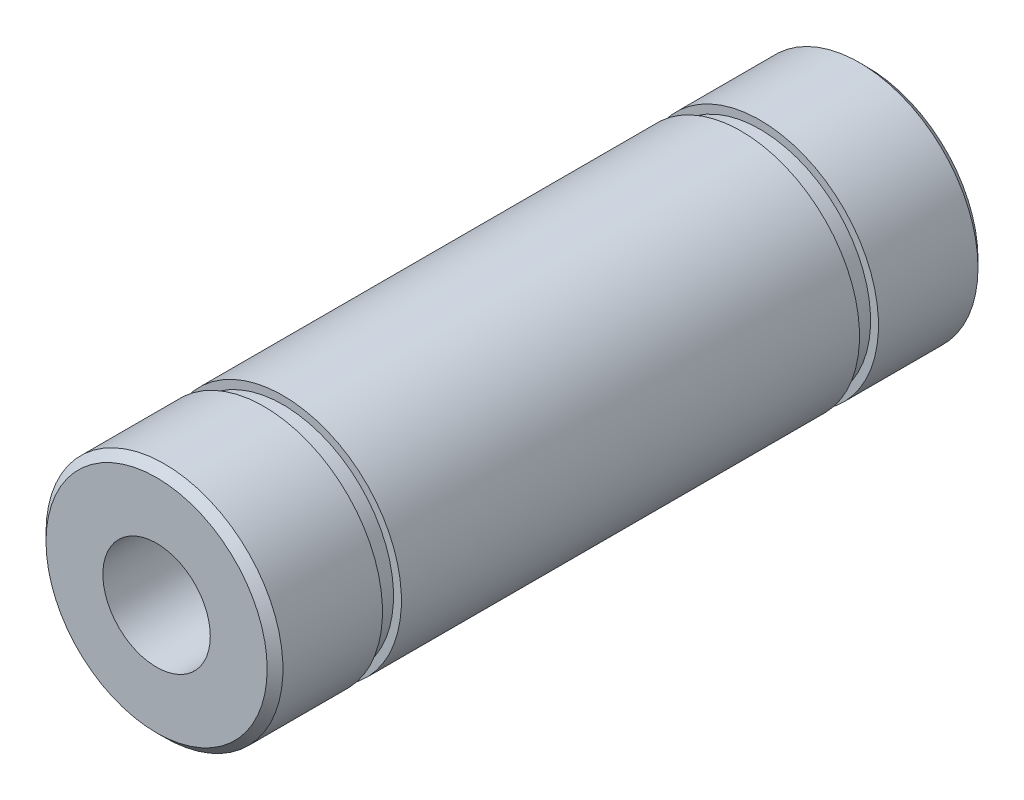
SolidWorks part; units mm, degrees
ref_plane "前视" through (0, 0, 0) normal (0, 0, 1) x (1, 0, 0)
ref_plane "上视" through (0, 0, 0) normal (0, 1, 0) x (1, 0, 0)
ref_plane "右视" through (0, 0, 0) normal (1, 0, 0) x (0, 0, -1)
sketch "草图1" plane through (0, 0, 0) normal (0, 0, 1) x (1, 0, 0)
  circle A0 centre (0, 0) radius 7.5
  dimension "D1" = 15
extrude "凸台-拉伸1" add sketch "草图1" along normal mid plane 45
hole_wizard "M8 螺纹孔1" positions "草图3" profile "草图2" tap size "M8" standard "Iso"
sketch "草图3" plane through (0, 0, 22.5) normal (0, 0, 1) x (1, 0, 0)
  point P0 (0, 0)
sketch "草图2" plane through (0, 0, 22.5) normal (1, 0, 0) x (0, -1, 0)
  line L0 (0, 0) -> (0, 22.0429)
  line L1 (0, 22.0429) -> (3.4, 20)
  line L2 (3.4, 20) -> (3.4, 0)
  line L5 (3.4, 0) -> (0, 0)
  line L10 (0, 22.0429) -> (-3.4, 20) construction
  line L11 (0, -6.35) -> (0, 107.95) construction
  dimension "螺纹孔钻头直径" = 6.8
  dimension "螺纹孔钻头深度" = 20
  dimension "导头角度" = 118
cosmetic thread "孔螺蚊线1" parameters "D1"=16, "D2"=8
chamfer "倒角1" distance 0.5 angle 45 2 edges at (7.5, 0, 22.5) (7.5, 0, -22.5)
mirror "镜向3" about plane through (0, 0, 0) normal (0, 0, 1) of "M8 螺纹孔1"
sketch "草图4" plane through (0, 0, 0) normal (0, 1, 0) x (1, 0, 0)
  line L0 (7.5, -22) -> (7.5, 22) construction
  line L1 (7.5, 15.7) -> (7, 15.7)
  line L2 (7.5, 15.7) -> (7.5, 14.5)
  line L3 (7.5, 14.5) -> (7, 14.5)
  line L4 (7, 15.7) -> (7, 14.5)
  line L5 (-13.0924, 0) -> (11.5905, 0) construction
  line L6 (0, 24.6885) -> (0, -27.9722) construction
  dimension "D1" = 1.2
  dimension "D2" = 14
  dimension "D3" = 29
revolve "切除-旋转1" cut sketch "草图4" angle 360 about L6
mirror "镜向5" about plane through (0, 0, 0) normal (0, 0, 1) of "切除-旋转1"
